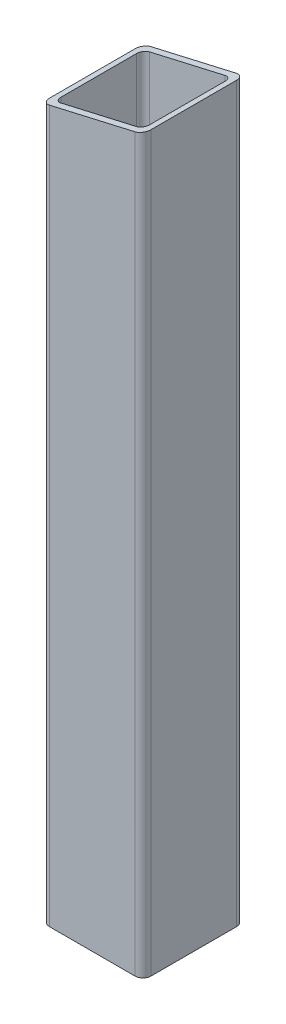
SolidWorks part; units mm, degrees
material "Angle steel 100×100×6/Q235"
ref_plane "Front Plane" through (0, 0, 0) normal (0, 0, 1) x (1, 0, 0)
ref_plane "Top Plane" through (0, 0, 0) normal (0, 1, 0) x (1, 0, 0)
ref_plane "Right Plane" through (0, 0, 0) normal (1, 0, 0) x (0, 0, -1)
sketch "Sketch2" plane through (0, 0, 0) normal (0, 1, 0) x (1, 0, 0)
  line L0 (12.6, 4.775) -> (87.4, 4.775)
  line L1 (6.3, 11.075) -> (6.3, 85.875)
  line L2 (87.4, 92.175) -> (12.6, 92.175)
  line L3 (93.7, 85.875) -> (93.7, 11.075)
  line L4 (7.875, -1.525) -> (92.125, -1.525)
  line L5 (0, 6.35) -> (0, 90.6)
  line L6 (92.125, 98.475) -> (7.875, 98.475)
  line L7 (100, 90.6) -> (100, 6.35)
  arc A0 (100, 90.6) -> (92.125, 98.475) centre (92.125, 90.6) ccw
  arc A1 (92.125, -1.525) -> (100, 6.35) centre (92.125, 6.35) ccw
  arc A2 (0, 6.35) -> (7.875, -1.525) centre (7.875, 6.35) ccw
  arc A3 (7.875, 98.475) -> (0, 90.6) centre (7.875, 90.6) ccw
  arc A4 (12.6, 92.175) -> (6.3, 85.875) centre (12.6, 85.875) ccw
  arc A5 (93.7, 85.875) -> (87.4, 92.175) centre (87.4, 85.875) ccw
  arc A6 (87.4, 4.775) -> (93.7, 11.075) centre (87.4, 11.075) ccw
  arc A7 (6.3, 11.075) -> (12.6, 4.775) centre (12.6, 11.075) ccw
extrude "Boss-Extrude1" add sketch "Sketch2" along normal mid plane 723
sketch "Sketch4" plane through (0, 0, 1.525) normal (0, 0, 1) x (1, 0, 0)
  line L0 (100, 361.5) -> (0, 338.5)
  line L1 (0, 361.5) -> (0, -361.5) construction
  line L2 (0, 338.5) -> (0, 361.5)
  line L3 (0, 361.5) -> (100, 361.5)
  line L4 (7.875, -361.5) -> (92.125, -361.5) construction
  dimension "D1" = 23
  dimension "D2" = 700
extrude "Cut-Extrude1" cut sketch "Sketch4" against normal up to next
